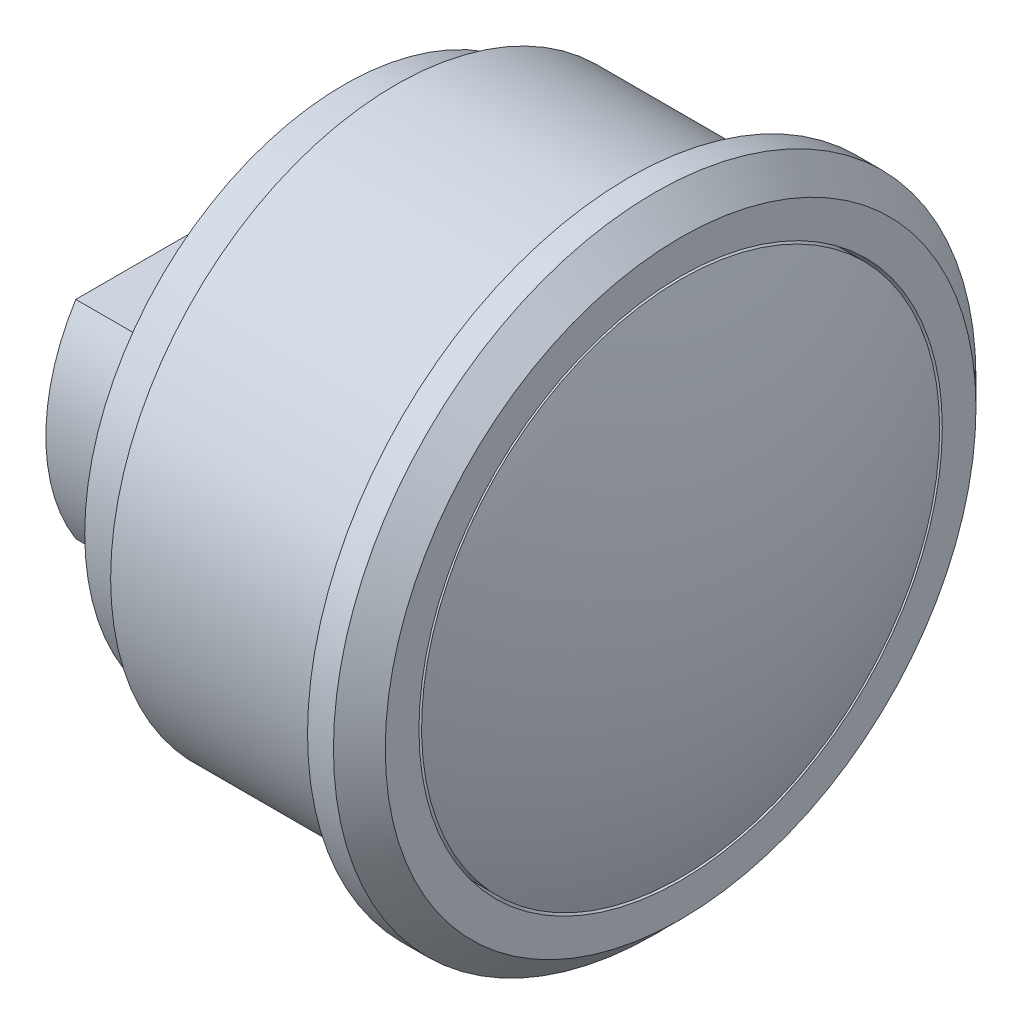
SolidWorks part; units mm, degrees
other "细节项目1"
ref_plane "Front Plane" through (0, 0, 0) normal (0, 0, 1) x (1, 0, 0)
ref_plane "Top Plane" through (0, 0, 0) normal (0, 1, 0) x (1, 0, 0)
ref_plane "Right Plane" through (0, 0, 0) normal (1, 0, 0) x (0, 0, -1)
sketch "Sketch1" plane through (0, 0, 0) normal (0, 1, 0) x (1, 0, 0)
  line L0 (0, 0) -> (17, 0)
  line L1 (17, 0) -> (17, 12.4)
  line L2 (17, 12.4) -> (15, 12.4)
  line L3 (15, 12.4) -> (15, 11)
  line L4 (15, 11) -> (6, 11)
  line L5 (6, 11) -> (6, 10)
  line L6 (6, 10) -> (4, 10)
  line L7 (4, 10) -> (4, 7.5)
  line L8 (4, 7.5) -> (0, 7.5)
  line L9 (0, 7.5) -> (0, 0)
  dimension "D1" = 12.4
  dimension "D2" = 2
  dimension "D3" = 9
  dimension "D4" = 11
  dimension "D5" = 10
  dimension "D6" = 13
  dimension "D7" = 7.5
  dimension "D8" = 4
revolve "Revolve1" add sketch "Sketch1" angle 360 about L0
sketch "Sketch2" plane through (17, 0, 0) normal (1, 0, 0) x (0, 0, -1)
  circle A0 centre (0, 0) radius 5.75
  dimension "D1" = 11.5
sketch "Sketch3" plane through (0, 0, 0) normal (0, 0, 1) x (1, 0, 0)
  line L0 (0, 0) -> (17, 0) construction
  line L1 (17, -5.75) -> (17, 5.75) construction
  line L2 (0, 0) -> (19, 0) construction
  line L3 (9, 0) -> (9, 10)
  line L4 (9, 0) -> (19, 0)
  line L5 (9, 10) -> (17, 10)
  line L6 (17, -12.4) -> (17, 12.4) construction
  line L7 (9, -10) -> (17, -10) construction
  arc A1 (19, 0) -> (17, 10) centre (-7, 0) ccw
  dimension "D2" = 8
revolve "Revolve2" add sketch "Sketch3" angle 360 about L4
sketch "Sketch4" plane through (0, 0, 0) normal (0, 1, 0) x (1, 0, 0)
  line L0 (0, 0) -> (19, 0) construction
chamfer "Chamfer1" distance 1 angle 45 1 edges at (17, 0, 12.4)
sketch "Sketch5" plane through (0, 0, 0) normal (-1, 0, 0) x (0, 0, 1)
  line L1 (-8.4009, 4) -> (8.4009, 4)
  line L2 (-8.4009, 4) -> (-8.4009, -4)
  line L3 (-8.4009, -4) -> (8.4009, -4)
  line L4 (8.4009, 4) -> (8.4009, -4)
  line L5 (-8.4009, 4) -> (8.4009, -4) construction
  line L6 (-8.4009, -4) -> (8.4009, 4) construction
  point P0 (0, 0)
  dimension "D1" = 8
extrude "Cut-Extrude2" cut sketch "Sketch5" against normal up to surface (4 mm away) flip side to cut up to face at (4, 0, 7.5)
sketch "Sketch7" plane through (17, 0, 0) normal (1, 0, 0) x (0, 0, -1)
  circle A0 centre (0, 0) radius 10
  circle A1 centre (0, 0) radius 10.1
  dimension "D1" = 20.2
extrude "Cut-Extrude3" cut sketch "Sketch7" against normal blind 3
